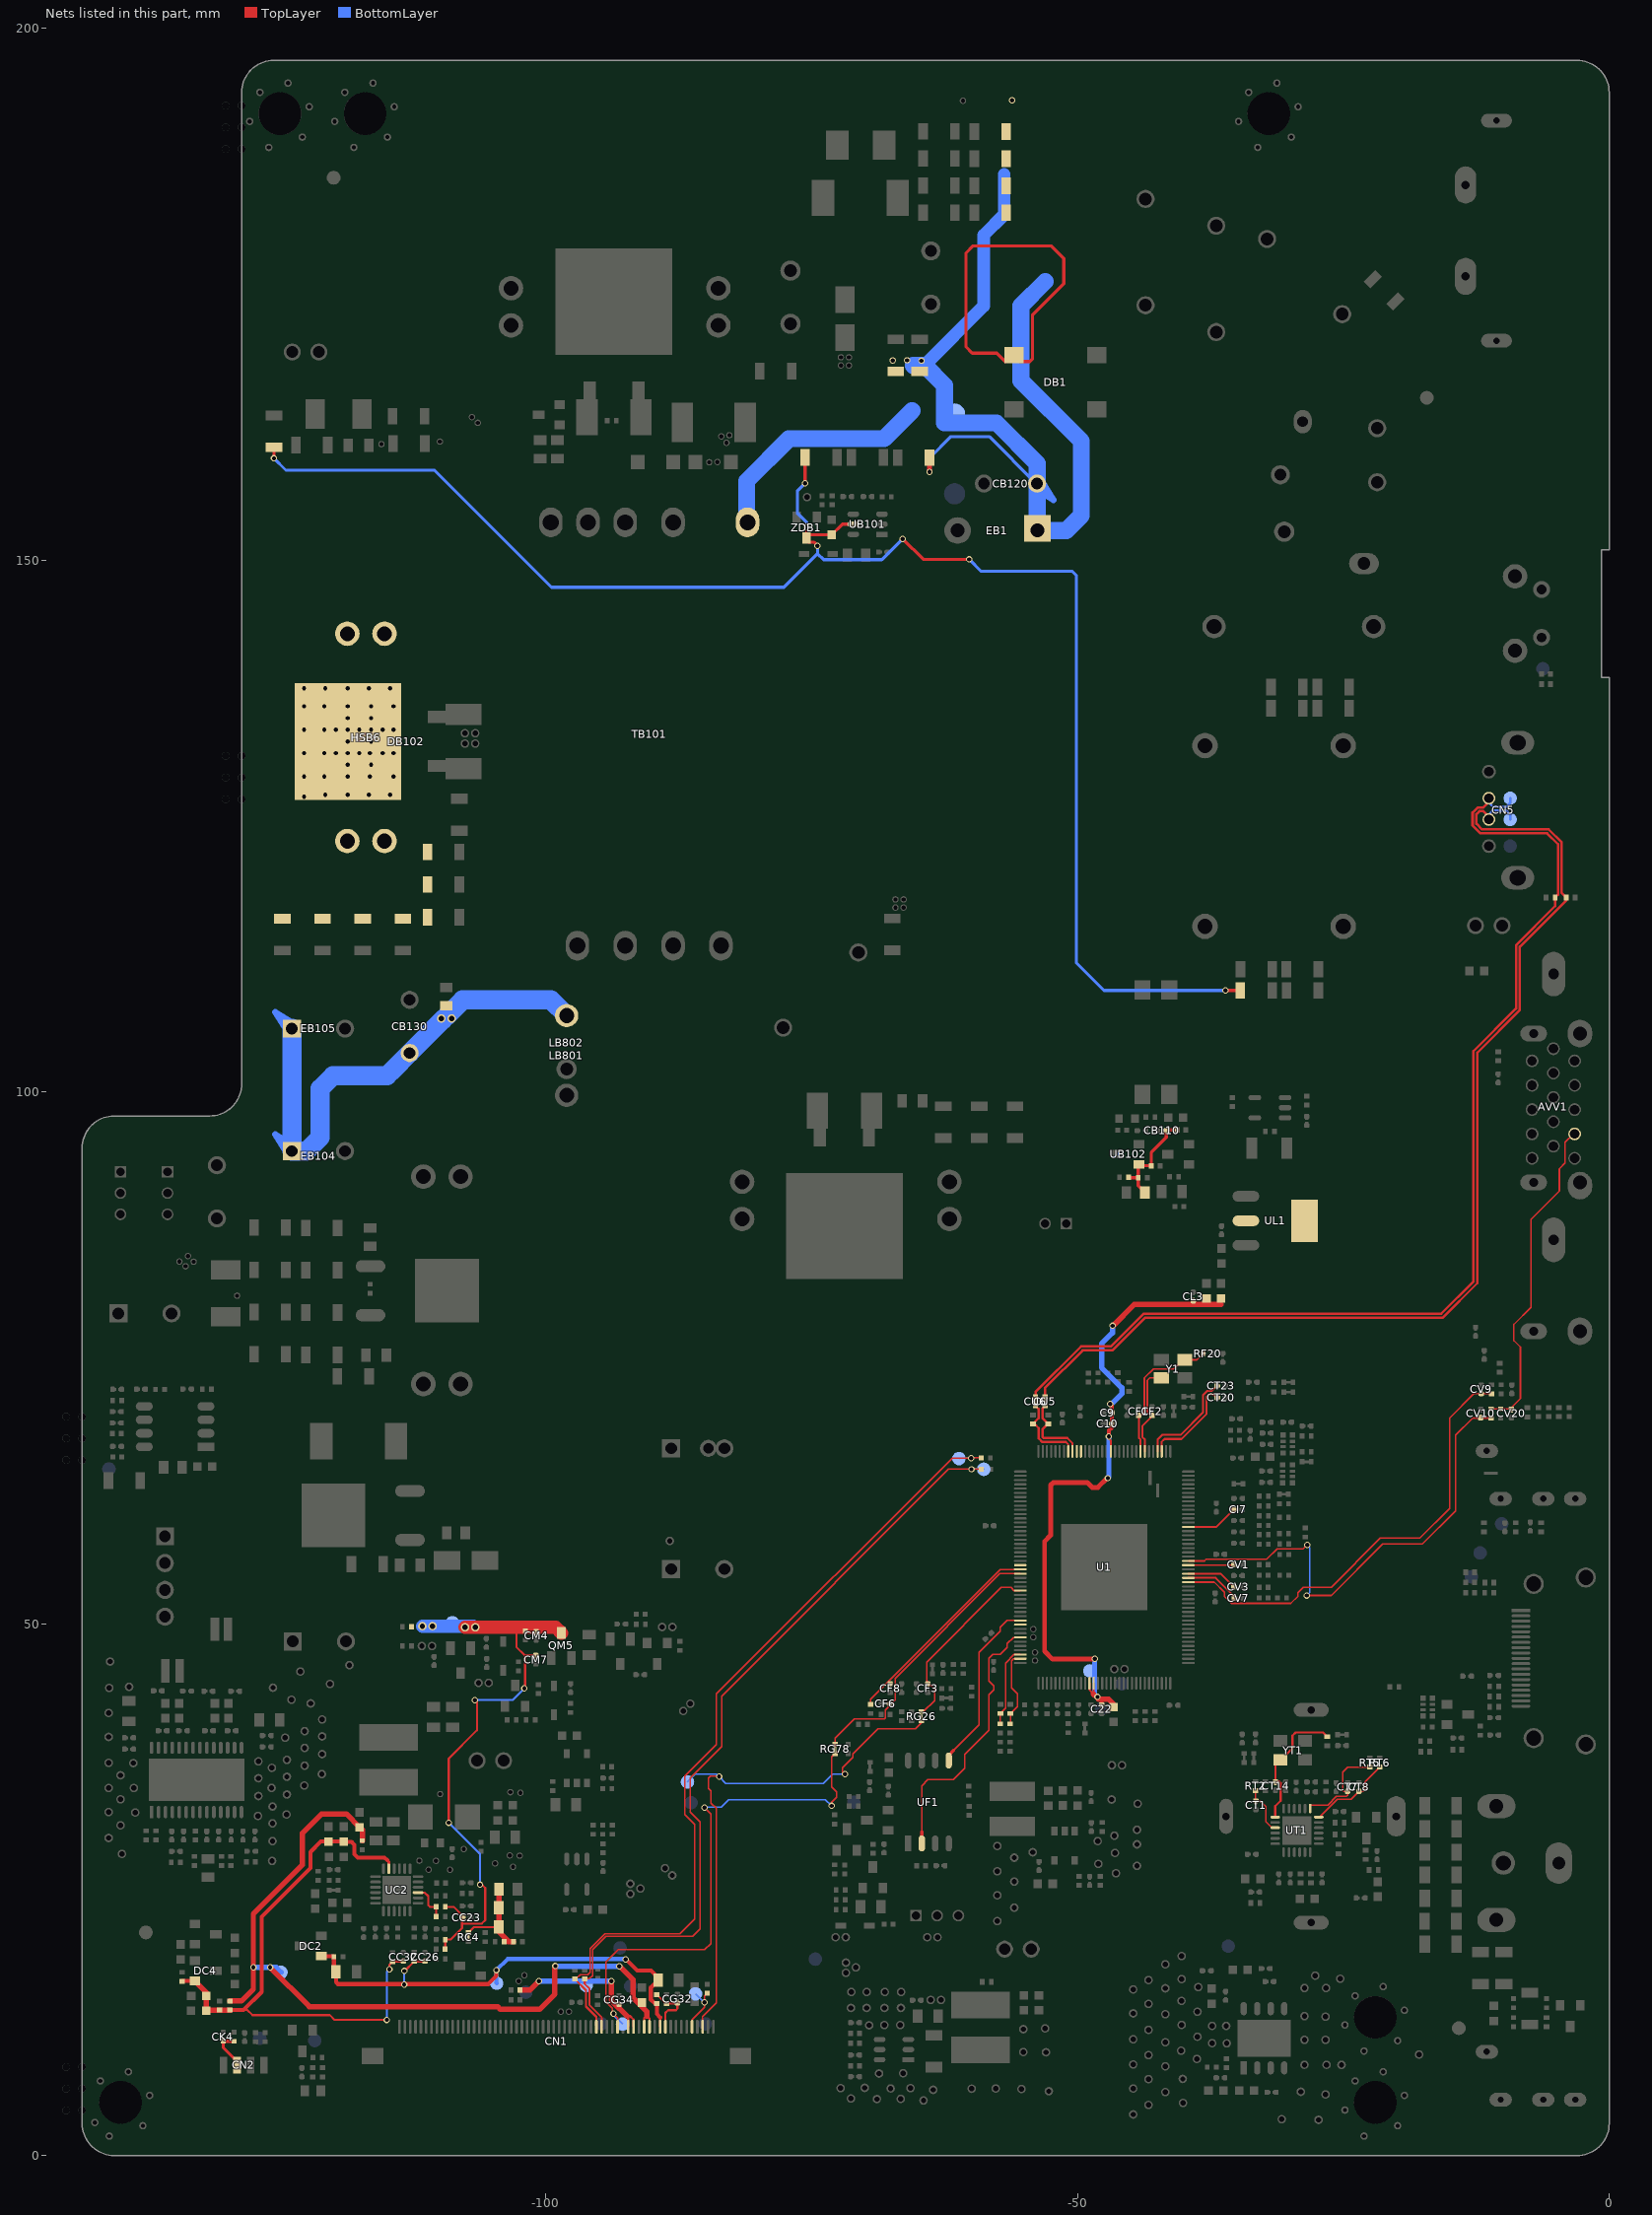
[diagram p0: the nets of this part, all layers, seen from the top]
# Altium PCB MISC86383-9.PcbDoc (part 15 of 18)
Units mm, origin at the board's own origin, x right, y up, seen from the top; angles counter-clockwise.
Board outline 143.6 x 197 mm, 2 copper layers (TopLayer, BottomLayer), stack 1.571 mm thick; 743 components, 401 nets, 2996 pads, 1077 vias.
Unrouted connection lines stored in the file: 4.

## Via types
v1: diameter 0.6, hole 0.4, TopLayer to BottomLayer, tented both sides, 993 vias
v2: diameter 0.6, hole 0.4, TopLayer to BottomLayer, 65 vias
v3: diameter 0.7, hole 0.5, TopLayer to BottomLayer, tented both sides, 15 vias
v4: diameter 0.8, hole 0.5, TopLayer to BottomLayer, tented both sides, 4 vias

## Nets (pads, with @x,y where several pads share a name; then routed paths per layer and width w, separated by ;. In a path a pad name is that pad's centre, name@x,y a point inside that pad or via, vN(x,y) a via of type N, cw(c..) or ccw(c..) an arc to the next point about the centre after c; other vN are vias at no path point) (continued)
SPI_SDI: U1.114 UF1.5 | length 16.7
  TopLayer w0.127: UF1.5@-62.106,37.142 UF1.5@-62.106,37.636 ; -61.671,38.08 -61.662,38.08 -59.245,40.497 -59.245,47.328 -57.262,49.312 -57.262,49.661 -56.61,50.313 U1.114@-55.371,50.313
  TopLayer w0.305: UF1.5@-62.106,37.636 -62.106,37.645 -61.671,38.08
SPI_SDO: U1.118 UF1.2 | length 25.8
  TopLayer w0.127: -64.646,30.449 -64.646,34.77 -64.071,35.344 -61.648,35.344 -60.592,36.4 -60.592,37.714 -58.331,39.974 -58.331,43.308 -57.858,43.781 -57.858,44.172 -58.331,44.645 -58.331,46.757 -57.944,47.144 -57.25,47.144 -56.602,47.792 -56.602,48.142 -56.031,48.713 U1.118@-55.371,48.713
  TopLayer w0.305: UF1.2@-64.646,29.342 -64.646,30.449
SPI_WP: U1.115
STV: CN1.58 RG26.2 RG26.3 STV.1 | length 51.5
  TopLayer w0.127: CN1.58@-85.25,12.103 -85.25,13.064 -83.972,14.342 -83.972,32.669 -84.45,33.148 -84.45,34.277 -84.691,34.519 -84.691,35.501 -84.525,35.668 -84.032,35.668 -84.026,35.674 -83.795,35.674 -83.718,35.598 -83.718,35.608 v1(-83.7,35.626) ; v1(-71.857,35.865) -71.869,35.852 -72.022,35.852 -72.098,35.928 -72.098,36.462 -71.133,37.427 -71.133,37.724 ; -71.124,37.724 -71.124,37.756 -68.757,40.123 -65.236,40.123 -64.694,40.665 RG26.2@-64.694,40.875
  BottomLayer w0.127: STV.1@-86.677,35.128 -85.941,35.865 -83.939,35.865 v1(-83.7,35.626) -83.063,34.989 -73.882,34.989 -73.006,35.865 v1(-71.857,35.865)
STV/: CF3.1 RG26.1 U1.107 | length 17.4
  TopLayer w0.127: RG26.1@-64.694,41.725 -64.503,41.725 -63.449,42.779 -63.449,43.878 -63.918,44.347 -64.006,44.435 -64.186,44.615 -64.186,46.388 -57.169,53.405 -56.253,53.405 -55.961,53.113 U1.107@-55.371,53.113
STY: CB110.2@-41.637,96.393 CB110.2@-41.812,96.393 RB133.1 RB134.2 RB135.2 RB180.2 RB181.2 UB102.R | length 9.7
  TopLayer w0.3: RB135.2@-45.193,91.973 -45.168,91.948 RB134.2@-44.291,91.948 ; RB181.2@-43.66,90.551 -44.291,91.182 RB134.2@-44.291,91.948 ; RB133.1@-40.659,96.444 -41.586,96.444 CB110.2@-41.637,96.393 -41.637,95.726 -43.072,94.292 RB180.2@-43.072,93.066 -44.082,93.066 -44.291,92.856 RB134.2@-44.291,91.948
T-IF-AGC: CT1.2@-33.225,33.183 CT1.2@-33.225,33.358 RT2.1 UT1.15 | length 4.7
  TopLayer w0.152: CT1.2@-33.259,33.358 -33.259,34.31 RT2.1@-33.258,34.311 ; CT1.2@-33.225,33.358 -32.812,33.358 -32.273,32.819 -32.273,31.392 -31.701,30.82 UT1.15@-31.41,30.82
TCON6: CF8.1 RG62.1 U1.102 | length 19.6
  TopLayer w0.127: RG62.1@-69.469,42.411 -69.469,42.901 -67.809,44.561 -57.257,55.113 U1.102@-55.371,55.113
TCON7: U1.101
TP: CN1.42 RG78.2 RG78.3 TP.1 | length 49.4
  TopLayer w0.127: v1@-93.751,13.284 v1@-93.688,13.348 ; v1(-93.629,13.348) v1@-93.688,13.348 ; CN1.42@-93.25,12.103 -93.25,12.91 v1@-93.688,13.348 ; v1(-85.065,32.703) -84.48,32.118 -84.48,30.557 -84.48,20.285 -84.48,19.932 -85.062,19.35 -93.185,19.35 -94.348,18.186 -94.348,14.427 -93.751,13.83 -93.751,13.411 v1@-93.688,13.348 ; v1@-73.152,33.172 -72.636,33.688 -72.636,34.176 -73.114,34.653 -73.114,37.472 RG78.2@-72.784,37.802
  BottomLayer w0.127: v1(-93.629,13.348) -93.629,13.2 TP.1@-92.786,12.357 ; v1(-85.065,32.703) -84.988,32.779 -83.477,32.779 -82.791,33.465 -73.711,33.465 v1(-73.127,32.88) v1@-73.177,32.88
TP/: CF6.1 RG78.1 U1.103 | length 26
  TopLayer w0.127: RG78.1@-72.784,38.652 -72.784,39.227 -70.973,41.038 -68.168,41.038 -68.047,41.159 -68.047,41.91 -67.642,42.314 -67.622,42.335 -67.622,42.367 -67.571,42.418 -67.149,42.84 -67.149,44.861 -57.298,54.713 U1.103@-55.371,54.713
TUNER_SCL: CT8.2@-23.53,34.223 CT8.2@-23.53,34.398 RT6.1 UT1.6 | length 8.1
  TopLayer w0.127: UT1.6@-27.31,31.82 -27.23,31.82 -25.559,33.492 -24.279,33.492 -23.549,34.223 CT8.2@-23.53,34.223 -23.147,34.223 -22.992,34.377 -22.992,35.11 RT6.1@-21.581,36.521 RT6.1@-21.566,36.506
TUNER_SDA: CT7.2@-24.597,34.223 CT7.2@-24.597,34.398 RT5.1 UT1.7 | length 9.4
  TopLayer w0.127: UT1.7@-28.11,32.62 -28.11,32.875 -28.039,32.946 -26.464,32.946 -25.644,33.766 -24.717,33.766 -24.597,33.885 CT7.2@-24.597,34.223 ; CT7.2@-24.8,34.223 -24.959,34.223 -25.038,34.301 -25.038,36.057 -24.569,36.527 -22.501,36.527 RT5.1@-22.496,36.521 RT5.1@-22.596,36.521
TVCOM: CG34.2@-93.116,14.193 CG34.2@-93.116,14.368 CN1.44 CN1.45 RC32.1 TVCOM.1 | length 15.6
  TopLayer w0.203: -92.54,13.134 -92.394,13.134 -92.089,13.134 -91.75,12.794 CN1.45@-91.75,12.103 ; CN1.44@-92.25,12.103 -92.25,13.046 -92.215,13.081
  TopLayer w0.508: RC32.1@-102.42,15.545 -101.503,15.545 v1(-100.642,16.405) ; v1(-93.828,16.383) -93.84,16.37 -93.84,14.58 -93.372,14.112 -93.285,14.024 -93.116,13.856 ; CG34.2@-93.116,14.193 -93.116,13.856 ; -92.394,13.134 -93.116,13.856
  BottomLayer w0.508: v1@-100.457,16.383 -96.202,16.383 v1(-93.828,16.383)
UART-RX/DDC: DV1.K RV19.1 U1.123 | length 7.4
  TopLayer w0.127: RV19.1@-56.348,40.587 -56.297,40.637 DV1.K@-56.297,41.565 -55.636,42.226 -55.636,43.413 -56.195,43.972 -56.195,46.511 -55.993,46.713 U1.123@-55.371,46.713
UART-TX/DDC: DV2.K RV18.1 U1.122 | length 7.7
  TopLayer w0.127: RV18.1@-57.262,40.587 DV2.K@-57.262,41.565 -56.762,42.065 -56.762,46.303 -55.952,47.113 U1.122@-55.371,47.113
USB0_DM: CN5.2@-11.31,125.63 CU5.1 DU4.K USB0_DM.1 | length 105.3
  TopLayer w0.234: CU5.1@-53.035,71.36 -53.055,71.36 -53.055,72.174 -49.517,75.711 -46.709,75.711 -43.624,78.796 -15.634,78.796 -12.403,82.027 -12.403,103.702 -8.396,107.709 -8.396,113.661 -4.049,118.007 DU4.K@-4.049,118.307 -4.456,118.713 -4.456,123.466 -5.68,124.69 -11.947,124.69 -12.483,125.225 -12.483,126.123 -12.196,126.41 -11.842,126.41 -11.31,125.877 CN5.2@-11.31,125.63
  BottomLayer w0.234: CN5.2@-11.31,125.63 -11.31,126.082 -10.914,126.479 -9.701,126.479 -9.31,126.088 USB0_DM.1@-9.31,125.63
USB0_DM/: CU5.2 CU5.3 DU2.K U1.70 | length 7.3
  TopLayer w0.178: -50.943,67.455 -50.471,66.983 U1.70@-50.471,66.213
  TopLayer w0.234: CU5.2@-53.035,70.482 -53.289,70.228 -53.289,69.342 DU2.K@-52.73,68.783 -52.8,68.783 -53.289,68.294 -53.289,67.591 -53.153,67.455 -50.943,67.455
USB0_DP: CN5.3@-11.31,127.63 CU6.1 DU3.K USB0_DP.1 | length 105.8
  TopLayer w0.234: CU6.1@-53.95,71.36 -53.95,71.789 -49.667,76.072 -46.858,76.072 -43.774,79.157 -15.783,79.157 -12.763,82.176 -12.763,103.851 -8.757,107.858 -8.757,113.81 -5.079,117.487 DU3.K@-5.079,118.305 -4.816,118.568 -4.816,123.316 -5.829,124.329 -12.096,124.329 -12.843,125.076 -12.843,126.272 -12.345,126.77 -11.824,126.77 -11.31,127.285 CN5.3@-11.31,127.63
  BottomLayer w0.234: CN5.3@-11.31,127.63 -11.31,127.219 -10.93,126.839 -9.644,126.839 -9.31,127.173 USB0_DP.1@-9.31,127.63
USB0_DP/: CU6.2 CU6.3 DU1.K U1.71 | length 7.4
  TopLayer w0.178: -51.093,67.095 -50.871,66.873 U1.71@-50.871,66.213
  TopLayer w0.234: CU6.2@-53.95,70.482 -53.65,70.182 -53.65,69.337 DU1.K@-54.204,68.783 -54.033,68.783 -53.65,68.4 -53.65,67.442 -53.303,67.095 -51.093,67.095
USB1_DM/: U1.68
USB1_DP/: U1.69
VBL: CB130.2 DB102.2 EB104.1@-123.874,94.45 EB105.1@-123.874,105.969 HSB6.1 HSB6.2 HSB6.3 HSB6.4 LB801.1@-98.044,107.191 LB802.1 pad.VIA5@-108.864,106.921 pad.VIA5@-109.83,106.921 RB124.2 RB125.2 RB126.2 RB127.2 RB140.1 RB162.2 RB163.2 RB164.2 | length 46.5
  BottomLayer w1.8: EB105.1@-123.874,105.969 -123.874,95.033 EB104.1@-123.874,94.45 -122.504,94.45 -121.221,95.733 -121.221,100.317 -120.002,101.536 -114.937,101.536 -114.357,102.116 CB130.2@-112.801,103.672 -109.691,106.783 -109.208,107.265 -107.812,108.661 -99.514,108.661 LB801.1@-98.044,107.191
  other v1: -122.733,127.767 -120.733,127.967 -118.633,127.967 -116.633,127.967 -114.633,127.967 -122.733,129.667 -120.833,129.667 -118.633,129.667 -116.533,129.667 -114.333,129.667 -118.633,130.767 -116.433,130.767 -122.733,131.867 -120.833,131.867 -119.733,131.867 -118.633,131.867 -117.533,131.867 -116.533,131.867 -115.333,131.867 -114.334,131.867 -118.633,132.967 -116.433,132.967 -122.733,134.067 -120.833,134.067 -119.733,134.067 -118.633,134.067 -117.533,134.067 -116.433,134.067 -115.333,134.067 -114.334,134.067 -118.633,135.167 -116.433,135.167 -122.734,136.267 -120.833,136.267 -118.633,136.267 -116.433,136.267 -114.333,136.267 -122.733,137.967 -120.733,137.967 -118.633,137.967 -116.633,137.967 -114.633,137.967
VBRIDGE: CB120.2 DB1.1 EB1.1@-53.775,152.801 pad.VIA5@-56.147,193.256 pad.VIA5@-64.668,168.77 pad.VIA5@-66.015,168.808 pad.VIA5@-67.373,168.796 RB117.2 RB118.2 RB143.2 RB150.2 RB151.2 RB152.2 RB156.2 TB101.1 TP-TDT.1 | length 151.9
  TopLayer w0.3: -60.49,177.749 -60.49,177.101 ; -57.389,169.282 -57.59,169.483 ; DB1.1@-56.808,168.701 -57.59,169.483 ; DB1.1@-55.97,169.301 -55.37,168.701 -54.46,168.701 -54.238,168.923 -54.238,173.053 -51.283,176.008 -51.283,178.371 -52.476,179.565 -59.804,179.565 -60.49,178.879 -60.49,177.101 ; -60.49,177.101 -60.49,170.08 -59.893,169.483 -57.59,169.483
  TopLayer w0.5: v2(-63.918,158.307) RB143.2@-63.918,159.664
  BottomLayer w0.3: v2(-63.918,158.307) -63.918,159.615 -61.9,161.633 -58.306,161.633 CB120.2@-53.886,157.213 ; CB120.2@-54.408,157.213 CB120.2@-53.886,157.213 ; CB120.2@-53.799,157.213 CB120.2@-53.886,157.213
  BottomLayer w1.2: -64.714,168.028 -64.429,168.313 -64.32,168.422 -58.826,173.916 -58.826,180.586 -56.896,182.516 -56.896,186.271
  BottomLayer w1.6: TB101.1@-81.028,153.567 -81.115,153.654 -81.115,157.455 -77.14,161.43 -68.199,161.43 -65.557,164.071 ; -65.443,168.313 -64.668,168.313 -64.429,168.313 -64.364,168.313 -62.497,166.446 -62.497,163.757 -62.497,162.916 -61.557,162.916 -57.62,162.916 -53.799,159.095 CB120.2@-53.799,157.213 -53.799,156.63 -53.799,152.825 EB1.1@-53.775,152.801 -51.047,152.801 -49.632,154.216 -49.632,161.214 -55.308,166.891 -55.308,170.167 ; -55.308,171.818 -55.308,170.167 ; -53.022,176.225 -55.308,173.939 -55.308,170.167
VCC: CB102.1 RB102.2 RB110.1 RB145.1 UB101.5 ZDB1.2 | length 153.3
  TopLayer w0.3: v2(-125.565,159.588) RB110.1@-125.565,160.615 ; v2(-75.616,157.251) -75.617,157.253 RB145.1@-75.617,159.677 RB145.1@-75.463,159.523 ; v2(-75.463,153.098) ZDB1.2@-75.463,152.094 -75.153,152.405 CB102.1@-73.114,152.405 -73.096,152.405 -72.111,153.391 UB101.5@-71.086,153.391 ; ZDB1.2@-75.298,151.714 -74.803,151.714 v2(-74.447,151.359) ; v2(-66.434,152.019) -64.503,150.089 v2(-60.185,150.089) ; v2(-36.081,109.563) RB102.2@-34.685,109.563
  BottomLayer w0.3: v2(-125.565,159.588) -124.447,158.471 -110.465,158.471 -99.466,147.472 -77.61,147.472 -74.447,150.635 ; v2(-75.616,157.251) -76.348,156.52 -76.348,154.461 -75.463,153.576 v2(-75.463,153.098) ; v2(-74.447,151.359) -74.447,150.635 ; v2(-66.434,152.019) -68.402,150.05 -73.863,150.05 -74.447,150.635 ; v2(-60.185,150.089) -59.068,148.972 -50.497,148.972 -50.104,148.579 -50.104,112.156 -47.511,109.563 v2(-36.081,109.563)
VCC_DDR: C9.2@-46.734,69.844 C9.2@-46.909,69.844 C10.2@-46.74,68.815 C10.2@-46.915,68.815 C11.2 C22.2@-47.725,42.228 C22.2@-47.725,42.403 CL3.2@-39.116,80.347 CL3.2@-39.116,80.522 CL4.2 CL5.2 U1.61 U1.137 U1.138 UL1.2 UL1.4 VCC_DDR.1 | length 64.5
  TopLayer w0.178: U1.137@-48.871,44.413 -48.871,43.771 -48.512,43.413 ; -48.471,43.613 U1.138@-48.471,44.413 ; v1@-47.07,67.429 -46.871,67.23 U1.61@-46.871,66.213
  TopLayer w0.305: C22.2@-47.743,42.314 C22.2@-47.725,42.314 ; C22.2@-47.725,42.403 -47.725,42.892 -47.712,42.905 ; C11.2@-46.84,41.994 C11.2@-46.658,42.176
  TopLayer w0.381: v1(-47.052,67.62) -47.052,68.178 -46.785,68.444 -46.785,68.815 -46.785,69.844 -46.785,70.515 v1(-46.937,70.667)
  TopLayer w0.457: v1(-48.372,46.71) -48.372,46.671 -52.339,46.671 -53.092,47.424 -53.092,57.752 -52.51,58.334 -52.51,63.042 -52.276,63.276 -49.071,63.276 -48.619,62.823 -48.076,62.823 v1@-47.204,63.695
  TopLayer w0.508: -48.512,43.413 -48.169,43.07 -48.004,42.905 -47.712,42.905 -47.052,42.905 -46.658,42.511 C11.2@-46.658,42.176 ; v1@-46.685,77.991 -44.641,80.035 -39.116,80.035 -37.871,80.035 -36.5,80.035
  BottomLayer w0.457: v1(-48.372,46.71) -48.377,46.705 -48.377,45.568 -48.377,43.379 v1(-48.119,43.121) ; v1(-47.141,63.695) -47.052,63.784 v1(-47.052,67.62)
  BottomLayer w0.508: v1(-46.937,70.667) -46.8,70.667 -45.837,71.63 -45.837,72.194 -47.737,74.093 -47.737,76.33 -46.711,77.356 v1(-46.711,78.016)
VCC_PANEL: CC23.2@-107.694,22.396 CC23.2@-107.869,22.396 CM4.1 CM7.2@-100.94,46.872 CM7.2@-100.94,47.047 pad.VIA5@-106.629,49.67 pad.VIA5@-107.594,49.67 pad.VIA5@-110.642,49.784 pad.VIA5@-111.608,49.784 QM5.D RC10.2 RC14.2 RC15.2 RC20.1 RM6.1 VCC_PANEL.1 | length 58.5
  TopLayer w0.203: RC10.2@-109.468,19.393 -109.455,19.406 RC14.2@-109.455,20.304 -108.94,20.304 -107.869,21.375 -107.869,21.806 ; RC15.2@-109.459,23.385 -108.666,23.385 -107.869,22.588 CC23.2@-107.869,22.396 -107.869,21.806 ; v1(-109.126,31.294) -109.126,37.33 -106.477,39.98 -106.477,42.824 v1(-106.68,42.824) ; v1(-106.185,25.463) -106.185,25.641 -106.096,25.552 -105.698,25.155 -105.698,22.127 -106.02,21.806 -107.869,21.806 ; -102.768,49.67 -102.768,47.822 -101.949,47.003 ; v1(-102.019,43.929) -101.949,43.999 -101.949,47.003 ; CM7.2@-100.94,47.047 -101.905,47.047 -101.949,47.003
  TopLayer w1.27: pad.VIA5@-107.594,49.67 pad.VIA5@-106.629,49.67 -102.768,49.67 -101.917,49.67 -100.902,49.67 -99.078,49.67 QM5.D@-98.54,49.131
  BottomLayer w0.203: v1(-109.126,31.294) -106.185,28.353 v1(-106.185,25.463) ; v1(-106.68,42.824) -103.124,42.824 v1(-102.019,43.929)
  BottomLayer w1.27: pad.VIA5@-111.595,49.771 -110.642,49.771 -108.788,49.771 -107.594,49.771 pad.VIA5@-106.832,49.771
VCOM: CI7.1 U1.33 | length 5
  TopLayer w0.178: U1.33@-39.571,59.113 -36.928,59.113 CI7.1@-35.307,60.734 CI7.1@-35.386,60.813
VDIV: RC12.2 RC15.1 UC2.15 | length 3.7
  TopLayer w0.203: UC2.15@-112.014,24.723 -111.388,24.723 -111.048,24.383 -111.048,23.545 -110.888,23.385 RC15.1@-110.309,23.385 RC12.2@-110.309,22.471
VGA_BIN: CV7.1 U1.21 | length 5.2
  TopLayer w0.18: U1.21@-39.571,54.313 -37.003,54.313 -35.295,52.605 CV7.1@-35.295,52.397
VGA_GIN: CV3.1 U1.22 | length 4.8
  TopLayer w0.18: U1.22@-39.571,54.713 -36.539,54.713 -35.308,53.481 CV3.1@-35.308,53.464
VGA_HS: CV9.2@-12.032,71.631 CV9.2@-12.032,71.806 RV6.2 U1.20 | length 43
  TopLayer w0.152: U1.20@-39.571,53.913 -37.136,53.913 -36.182,52.959 -36.182,52.565 -35.537,51.92 -29.939,51.92 -29.281,52.578 -29.281,52.912 -28.755,53.439 -26.131,53.439 -21.519,58.052 -19.576,58.052 -17.797,58.052 -14.998,60.85 -14.998,69.354 -12.721,71.631 CV9.2@-12.032,71.631 RV6.2@-11.067,71.631 RV6.2@-11.017,71.631
VGA_RIN: CV1.1 U1.24 | length 4.3
  TopLayer w0.18: U1.24@-39.571,55.513 -35.342,55.513 CV1.1@-35.308,55.547
VGA_VS: CV10.2@-12.084,69.35 CV10.2@-12.084,69.525 RV10.2 U1.25 | length 45.2
  TopLayer w0.152: U1.25@-39.571,55.913 -38.055,55.913 -37.882,56.086 -32.189,56.086 -31.219,57.056 -28.794,57.056 -28.443,57.406 v1(-28.392,57.406) ; v1(-28.431,52.657) -26.124,52.657 -21.287,57.493 -19.345,57.493 -17.565,57.493 -14.44,60.619 -14.44,67.741 -12.831,69.35 CV10.2@-12.084,69.35 -11.272,69.35 RV10.2@-11.119,69.35 RV10.2@-11.068,69.35
  BottomLayer w0.152: v1(-28.431,52.657) -28.147,52.94 -28.147,57.161 v1(-28.392,57.406)
VGH: CC9.1 CC10.1 CC32.2@-113.392,18.244 CC32.2@-113.392,18.419 CC33.2 CC34.2 DC4.3 RC23.2 RC27.2 RG5.2 RG9.2 UC2.23 | length 56
  TopLayer w0.203: -128.417,13.672 -128.054,13.672 -127.572,13.19 -120.309,13.19 -119.871,12.753 -114.948,12.753 v1@-114.946,12.753 ; v1(-114.948,12.751) v1@-114.946,12.753 ; v1@-114.897,12.753 v1@-114.946,12.753 ; v1@-114.706,17.361 v1(-114.706,17.501) -114.706,17.931 RG9.2@-114.399,18.239 ; RG9.2@-114.394,18.244 CC32.2@-113.392,18.244
  TopLayer w0.254: -114.91,27.762 -114.764,27.617 UC2.23@-114.764,26.973
  TopLayer w0.381: RC23.2@-134.212,16.378 -134.174,16.416 DC4.3@-133.005,16.416 ; RG5.2@-129.68,13.697 -129.673,13.691 -129.654,13.672 -128.417,13.672 -126.713,15.376 -126.713,22.461 -122.146,27.028 -122.146,28.541 -121.168,29.52 CC10.1@-120.421,29.52 CC9.1@-118.999,29.52 ; CC9.1@-118.991,29.477 -118.262,29.477 -118,29.214 -118,28.331 -117.684,28.016 -115.164,28.016 -114.91,27.762
  TopLayer w0.508: DC4.3@-133.005,16.416 -131.932,15.343 CC33.2@-131.932,15.011 CC34.2@-131.932,13.627 ; CC34.2@-131.945,13.614 CC34.2@-131.932,13.627 ; RG5.2@-129.654,13.672 RG5.2@-129.692,13.672 RC27.2@-130.683,13.672 -131.887,13.672 CC34.2@-131.932,13.627
  BottomLayer w0.203: v1(-114.948,12.751) -114.948,17.259 v1(-114.706,17.501)
VGHM: CG14.1 CG33.2 CN1.47 CN1.48 RG5.1 RG6.2 VON.1 | length 75.4
  TopLayer w0.203: CN1.47@-90.75,12.103 -90.75,12.933 -90.64,13.043 ; -90.373,13.005 -90.25,12.882 CN1.48@-90.25,12.103
  TopLayer w0.508: RG5.1@-129.692,14.522 -128.62,14.522 -127.505,15.637 v1(-127.503,17.682) -127.505,22.721 -122.89,27.336 -122.89,30.302 -121.076,32.116 -118.763,32.116 CG14.1@-117.5,30.853 -117.259,30.612 RG6.2@-117.259,29.61 ; v1(-125.92,17.682) -122.23,13.992 -104.537,13.992 -104.283,13.738 -100.586,13.738 -99.144,15.18 -99.144,17.772 v1(-99.098,17.818) ; v1(-93.078,17.793) -93.053,17.793 -91.783,16.523 -91.783,14.795 -91.163,14.176 -90.513,13.525 -90.513,13.119
  BottomLayer w0.508: v1(-127.503,17.682) v1(-125.92,17.682) -125.366,17.682 VON.1@-124.904,17.221 ; v1@-99.098,17.805 -93.078,17.805 -93.066,17.805 v1(-93.078,17.793)
VGL: CC26.2@-111.36,18.244 CC26.2@-111.36,18.419 CC29.1 CC30.1 CN1.50 DC2.1 RC24.2 RG21.2 RG39.1 VOFF.1 | length 46.3
  TopLayer w0.203: v1(-113.311,17.349) -113.271,17.349 RG21.2@-112.376,18.244 CC26.2@-111.36,18.244 ; CN1.50@-89.25,12.103 -89.25,12.999
  TopLayer w0.381: DC2.1@-121.101,18.752 -119.989,18.752 RC24.2@-119.932,18.694 -119.932,17.455 CC30.1@-119.736,17.259 -119.736,16.308 -119.552,16.123 -113.318,16.123 -105.403,16.123 -104.648,16.878 v1(-104.648,17.437) ; v1(-92.494,18.44) -92.494,18.479 -92.475,18.459 -91.415,17.399 -90.113,17.399 -89.434,16.72 CC29.1@-89.434,16.485 -90.128,15.791 -90.128,14.664 -89.745,14.282 RG39.1@-89.56,14.282 -89.56,13.31 -89.25,12.999
  BottomLayer w0.203: v1(-113.318,16.073) -113.311,16.081 v1(-113.311,17.349)
  BottomLayer w0.381: VOFF.1@-104.623,16.205 -104.648,16.231 v1(-104.648,17.437) -103.607,18.479 v1@-92.494,18.479
VIFM: CT23.2@-36.737,72.371 CT23.2@-36.912,72.371 U1.50 | length 9.7
  TopLayer w0.178: U1.50@-42.471,66.213 -42.471,67.32 -42.452,67.34
  TopLayer w0.203: -42.452,67.34 -42.032,67.759 -40.309,67.759 -38.191,69.877 -38.191,71.512 -37.806,71.897 -37.384,71.897 -36.912,72.369 CT23.2@-36.912,72.371
VIFP: CT20.2@-36.737,71.26 CT20.2@-36.912,71.26 U1.49 | length 9
  TopLayer w0.178: U1.49@-42.071,66.213 -42.071,67.126 -41.946,67.251
  TopLayer w0.203: -41.946,67.251 -41.819,67.378 -40.223,67.378 -37.86,69.74 -37.86,71.376 -37.669,71.567 -37.219,71.567 CT20.2@-36.912,71.26
VMID/I2C_SCL: CN1.39 RG42.2 RG60.2 VMID/SCL.1 | length 77.3
  TopLayer w0.127: RG42.2@-96.342,16.606 -95.904,16.606 -95.606,16.904 -95.606,19.342 -94.353,20.595 -86.2,20.595 -85.496,21.298 -85.496,31.345 -86.431,32.28 -86.431,35.471 -83.464,38.439 -83.464,43.184 -62.119,64.529 v1(-59.969,64.529) RG60.2@-59.036,64.529
  TopLayer w0.203: RG42.2@-96.342,16.606 -96.342,16.129 -95.885,15.672 -95.885,14.138 -94.75,13.003 CN1.39@-94.75,12.103
  BottomLayer w0.127: v1(-59.969,64.529) VMID/SCL.1@-58.814,64.529
VMID/I2C_SDA: CN1.38 RG43.2 RG61.2 VMID/SDA.1 | length 78.2
  TopLayer w0.127: RG43.2@-97.161,16.606 -96.771,16.996 -96.047,16.996 -95.834,17.209 -95.834,19.473 -94.458,20.849 -87.381,20.849 -86.004,22.225 -86.004,31.135 -86.939,32.07 -86.939,35.681 -83.972,38.649 -83.972,43.394 -61.783,65.583 v1(-59.995,65.583) -59.982,65.595 RG61.2@-59.048,65.595
  TopLayer w0.203: RG43.2@-97.161,16.606 -97.161,16.481 -96.215,15.535 -96.215,14.001 -95.25,13.036 CN1.38@-95.25,12.103
  BottomLayer w0.127: VMID/SDA.1@-61.15,65.532 -61.1,65.583 v1(-59.995,65.583)
VOFF: CG32.2@-87.617,14.32 CG32.2@-87.617,14.495 CN1.51 RG39.2 RG44.2 | length 5.4
  TopLayer w0.203: RG39.2@-89.56,15.132 -88.736,14.307 -88.633,14.307 -87.63,14.307 CG32.2@-87.617,14.32 -87.617,13.818 -87.77,13.665 -88.494,13.665 -88.75,13.409 CN1.51@-88.75,12.103
VREF: CC1.2 CC2.2 RC1.2 RC2.2 RC4.2 RC4.3 RG48.1 | length 8.9
  TopLayer w0.203: RC4.2@-107.29,20.948 -106.762,21.476 CC1.2@-104.42,21.476
  TopLayer w0.508: CC1.2@-104.42,21.483 -104.42,21.476 -104.42,21.037 -103.5,20.117 RG48.1@-103.041,20.117 ; CC1.2@-104.413,21.483 -104.413,25.028 RC1.2@-104.396,25.044
VS: CK4.1 CN2.2 RK13.2 | length 3.7
  TopLayer w0.305: RK13.2@-129.439,10.7 -129.487,10.749 CK4.1@-130.333,10.749 -130.333,10.145 -129.035,8.848 CN2.2@-129.035,8.505
VS_VGA: AVV1.14 CV20.2@-9.195,70.031 CV20.2@-9.195,70.206 RV10.1 RV14.1 | length 30.7
  TopLayer w0.152: RV10.1@-11.068,70.2 RV14.1@-10.205,70.2 -9.341,70.2 -9.265,70.276 -8.352,71.189 -8.352,76.023 -8.957,76.628 -8.957,78.149 -7.341,79.766 -7.341,88.031 -4.686,90.686 -4.686,92.786 -4.141,93.331 -4.141,95.266 -3.297,96.11 AVV1.14@-3.247,96.16
XAO: CN1.56 RG41.2 XAO.1 | length 4.9
  TopLayer w0.127: CN1.56@-86.25,12.103 -86.25,12.783 -85.077,13.955 v1(-85.077,14.389) -85.077,14.993 RG41.2@-84.823,15.247
  BottomLayer w0.127: XAO.1@-85.915,15.202 -85.103,14.389 v1(-85.077,14.389)
XTAL_O: CT14.2@-31.379,34.986 CT14.2@-31.379,35.161 LF1.2 UT1.13 YT1.1 | length 12.5
  TopLayer w0.203: UT1.13@-31.41,31.82 -31.41,32.852 -30.9,33.361 -30.9,35.033 -31.028,35.161 CT14.2@-31.379,35.161 -31.379,36.731 YT1.1@-30.908,37.202 -30.875,37.202 -29.783,38.294 -29.783,39.474 -29.476,39.781 -26.909,39.781 LF1.2@-26.52,39.391
XTALI: CF2.2@-42.979,69.564 CF2.2@-42.979,69.739 U1.53 Y1.3 | length 8.7
  TopLayer w0.152: CF2.2@-42.979,69.564 -43.123,69.564 -43.138,69.58 -43.432,69.873 -43.432,72.881 -43.192,73.12 Y1.3@-42.106,73.12
  TopLayer w0.178: U1.53@-43.671,66.213 -43.671,67.355 -43.897,67.581 -43.897,68.599 -43.068,69.429 CF2.2@-43.068,69.475
XTALO: CF1.2@-44.249,69.552 CF1.2@-44.249,69.727 RF20.1 U1.54 Y1.1 | length 13.8
  TopLayer w0.152: CF1.2@-44.249,69.552 -44.153,69.552 -44.074,69.552 -43.711,69.916 -43.711,73.116 -42.863,73.965 -40.945,73.965 -40.09,74.82 Y1.1@-39.906,74.82 -38.769,74.82 -38.18,75.409 RF20.1@-38.18,75.417
  TopLayer w0.178: CF1.2@-44.153,69.552 -44.201,69.504 -44.202,69.503 -44.202,67.455 -44.071,67.324 U1.54@-44.071,66.213